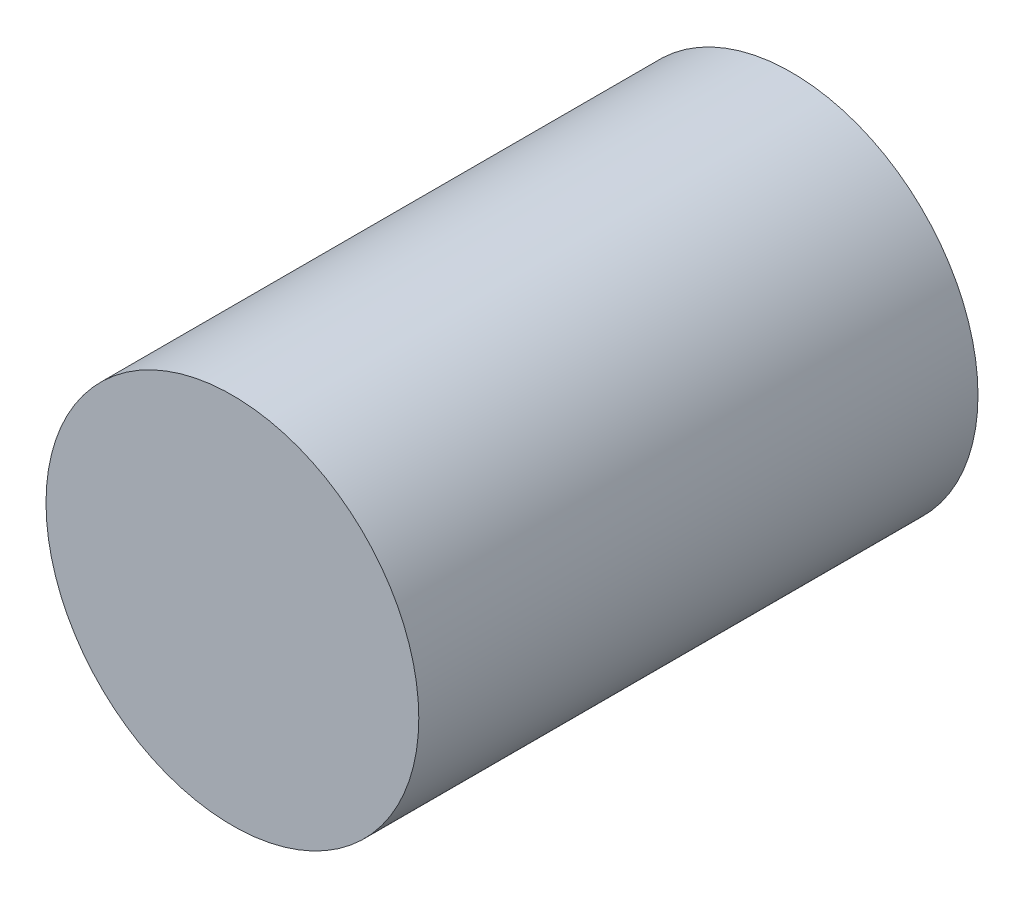
from build123d import *

# Parameters (mm, degrees)
SKETCH_1_R      = 4
EXTRUDE_1_DEPTH = 6


with BuildPart() as part:
    # 草图1 → 凸台-拉伸1 (new, symmetric)
    with BuildSketch(Plane.XY):
        Circle(SKETCH_1_R)
    extrude(amount=EXTRUDE_1_DEPTH, both=True)


solid = part.part
